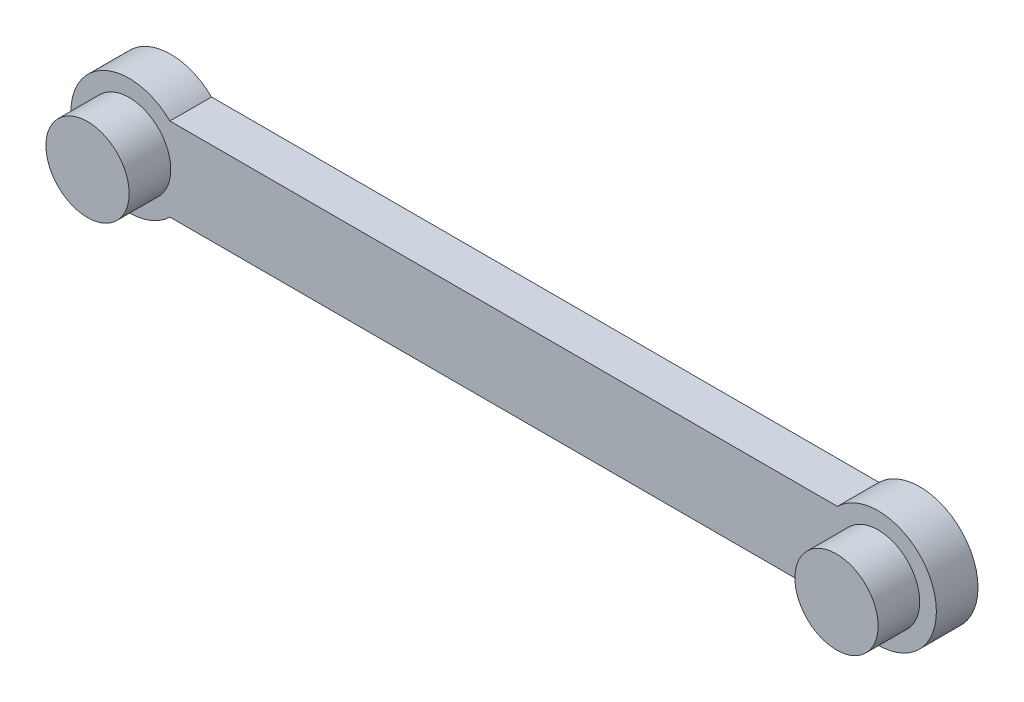
from build123d import *

# Parameters (mm, degrees)
BASE_EXTRUDE_DEPTH  = 5
SKETCH2_R           = 5
BOSS_EXTRUDE1_DEPTH = 5


with BuildPart() as part:
    # Sketch1 → Base-Extrude (new body)
    with BuildSketch(Plane.XY):
        with BuildLine():
            Line((4.898979486, -5), (85.101020514, -5))
            ThreePointArc((85.101020514, -5), (97, 0), (85.101020514, 5))
            Line((85.101020514, 5), (4.898979486, 5))
            ThreePointArc((4.898979486, 5), (-7, 0), (4.898979486, -5))
        make_face()
    extrude(amount=BASE_EXTRUDE_DEPTH)

    # Sketch2 → Boss-Extrude1 (add)
    with BuildSketch(Plane.XY.offset(5)):
        Circle(SKETCH2_R)
        with Locations((90, 0)):
            Circle(SKETCH2_R)
    extrude(amount=BOSS_EXTRUDE1_DEPTH)


solid = part.part
